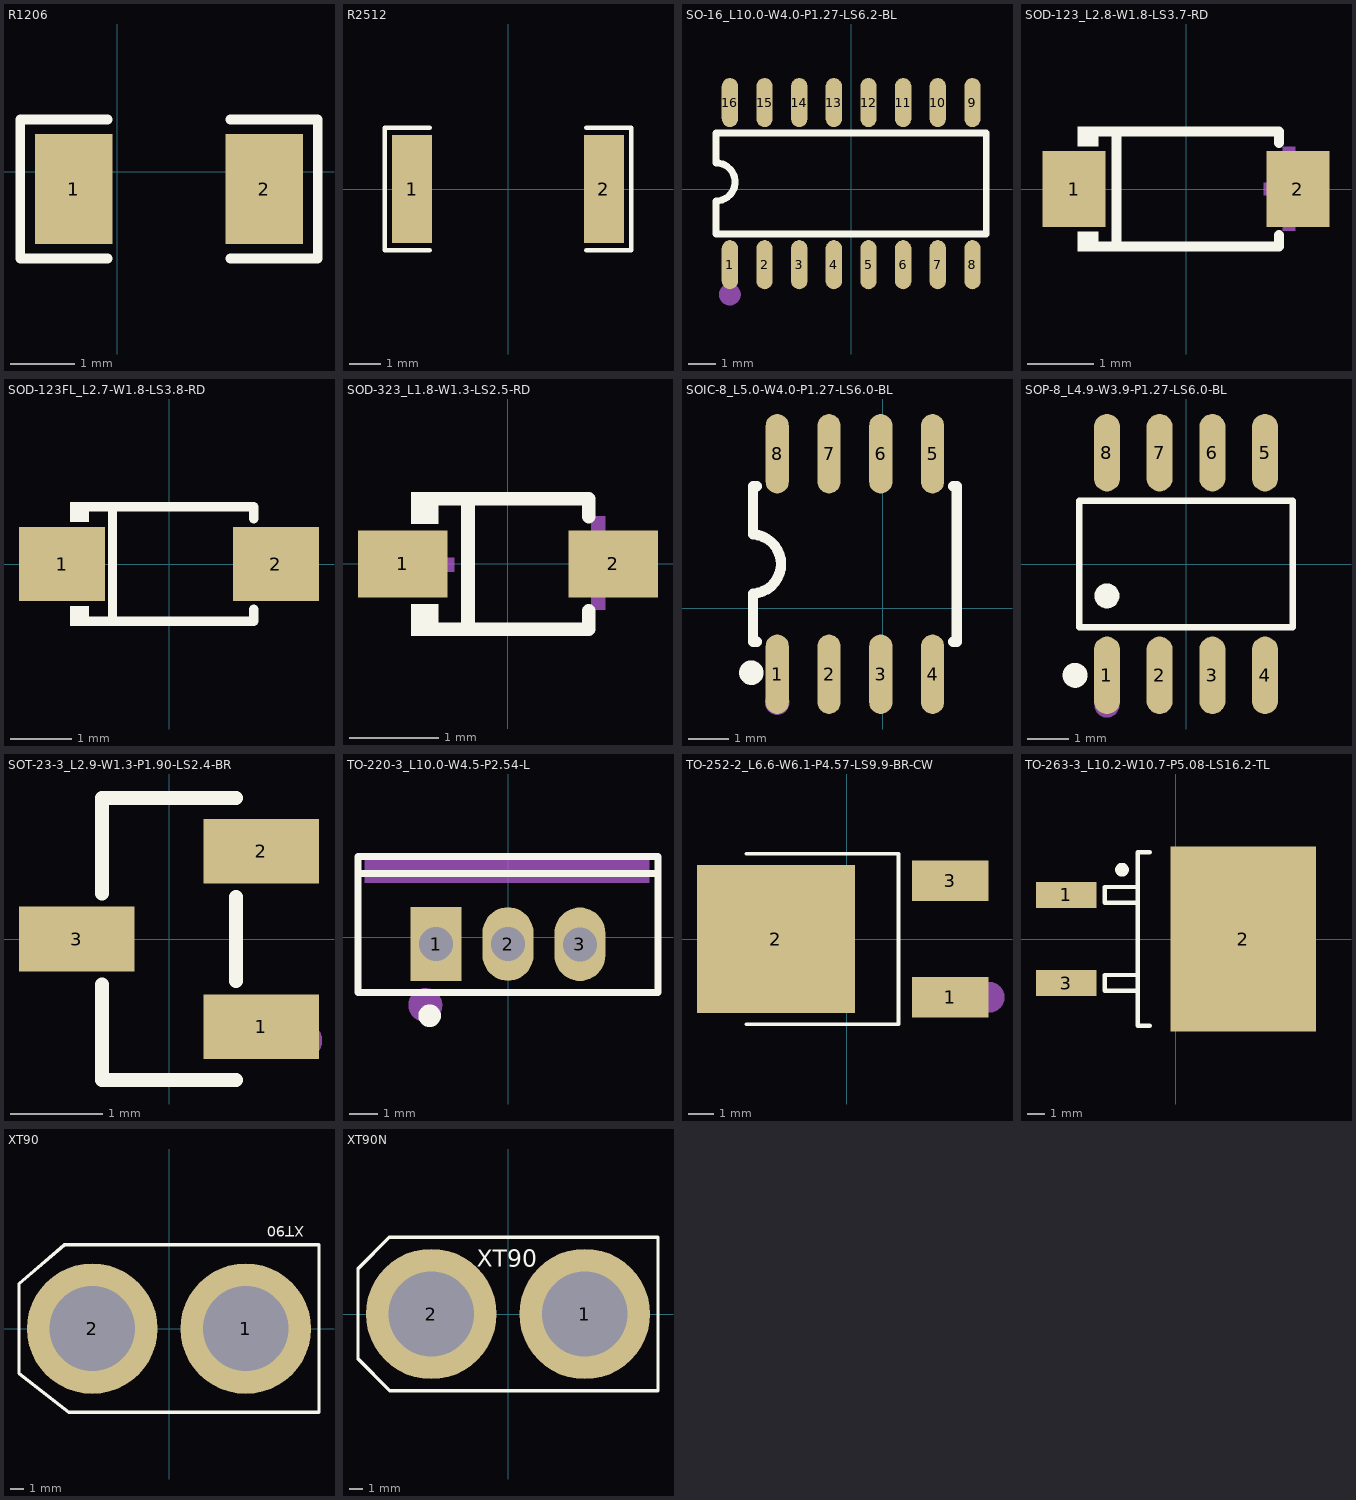
[diagram p0: the footprints below, top view; thin cyan lines are the x and y axes]
# Altium footprint library MISC84449-2.PcbLib: 30 footprints (part 2 of 2)
Each footprint in its own frame and in the unit in brackets; x right, y up, seen from the top. Pads: shape width x height; smd on the part's side, far side on the other; paste and mask are expansions set on the pad; w line width, h text height; cw(c..) or ccw(c..) is an arc to the next point about the centre after c.

## R1206 [mm]
pads (2):
  rect 1.208x1.701 smd: 1(-0.678,-0.267) 2(2.279,-0.267)
Top Overlay:
  lines w0.152: -0.151,-1.346 -1.511,-1.346 -1.511,0.812 -0.151,0.812 ; 1.751,-1.346 3.111,-1.346 3.111,0.812 1.751,0.812
Top Paste:
  region: -0.075,-1.017 -0.075,-0.656 -0.175,-0.556 -0.385,-0.556 -0.485,-0.456 -0.485,-0.078 -0.385,0.022 -0.175,0.022 -0.075,0.122 -0.075,0.484 -0.175,0.584 -1.182,0.584 -1.282,0.484 -1.282,-1.017 -1.182,-1.117 -0.175,-1.117
  region: 1.675,-1.017 1.675,-0.656 1.775,-0.556 1.986,-0.556 2.086,-0.456 2.086,-0.078 1.986,0.022 1.775,0.022 1.675,0.122 1.675,0.484 1.775,0.584 2.783,0.584 2.883,0.484 2.883,-1.017 2.783,-1.117 1.775,-1.117

## R2512 [mm]
pads (2):
  rect 1.283x3.456 smd: 1(-3.066,0) 2(3.066,0)
Top Overlay:
  lines w0.152: -2.501,-1.957 -3.936,-1.957 -3.936,1.957 -2.501,1.957 ; 2.501,-1.957 3.936,-1.957 3.936,1.957 2.501,1.957
Top Paste:
  region: 2.425,-1.628 2.425,-0.688 2.525,-0.588 2.761,-0.588 2.861,-0.488 2.861,0.488 2.761,0.588 2.525,0.588 2.425,0.688 2.425,1.628 2.525,1.728 3.608,1.728 3.708,1.628 3.708,-1.628 3.608,-1.728 2.525,-1.728
  region: -2.425,-1.628 -2.425,-0.688 -2.525,-0.588 -2.761,-0.588 -2.861,-0.488 -2.861,0.488 -2.761,0.588 -2.525,0.588 -2.425,0.688 -2.425,1.628 -2.525,1.728 -3.608,1.728 -3.708,1.628 -3.708,-1.628 -3.608,-1.728 -2.525,-1.728

## SO-16_L10.0-W4.0-P1.27-LS6.2-BL [mm]
pads (16):
  oval 0.6x1.8 smd: 1(-4.444,-2.776) 2(-3.174,-2.776) 3(-1.904,-2.776) 4(-0.634,-2.776) 5(0.636,-2.776) 6(1.906,-2.776) 7(3.176,-2.776) 8(4.446,-2.776) 9(4.446,3.168) 10(3.176,3.168) 11(1.906,3.168) 12(0.636,3.168) 13(-0.634,3.168) 14(-1.904,3.168) 15(-3.174,3.168) 16(-4.444,3.168)
Top Overlay:
  lines w0.254: -4.952,0.958 cw(c-4.952,0.26) -4.952,-0.439 -4.952,-1.654 -4.949,-1.654 4.952,-1.654 4.952,2.046 -4.949,2.046 -4.949,0.958
Mechanical 15:
  circle w0.4: c-4.444,-3.868 r0.2

## SOD-123_L2.8-W1.8-LS3.7-RD [mm]
pads (2):
  rect 0.95x1.15 smd: 1(-1.693,0) 2(1.693,0)
Top Overlay:
  region: -1.33,0.942 -1.33,0.647 -1.635,0.647 -1.635,0.942
  region: -1.33,-0.942 -1.33,-0.647 -1.635,-0.647 -1.635,-0.942
  lines w0.152: -1.406,-0.866 1.406,-0.866 1.406,-0.698 ; -1.406,0.866 1.406,0.866 1.406,0.698 ; -1.049,-0.866 -1.049,0.866
Mechanical 15:
  region: -2.03,0.095 -2.03,-0.095 -1.272,-0.095 -1.272,0.095
  region: 1.935,0.098 1.935,-0.092 1.177,-0.092 1.177,0.098
  region: 1.651,0.635 1.651,-0.629 1.461,-0.629 1.461,0.635

## SOD-123FL_L2.7-W1.8-LS3.8-RD [mm]
pads (2):
  rect 1.4x1.2 smd: 1(-1.735,0) 2(1.735,0)
Top Overlay:
  region: -1.3,1.002 -1.3,0.682 -1.605,0.682 -1.605,1.002
  region: -1.3,-1.002 -1.3,-0.682 -1.605,-0.682 -1.605,-1.002
  lines w0.152: -1.376,-0.926 1.376,-0.926 1.376,-0.733 ; -1.376,0.926 1.376,0.926 1.376,0.733 ; -0.917,-0.876 -0.917,0.876
Mechanical 15:
  region: -2.032,0.127 -2.032,-0.065 -1.264,-0.065 -1.264,0.127
  region: 2.035,0.096 2.035,-0.096 1.267,-0.096 1.267,0.096
  region: 1.747,-0.384 1.555,-0.384 1.555,0.384 1.747,0.384

## SOD-323_L1.8-W1.3-LS2.5-RD [mm]
pads (2):
  rect 1x0.75 smd: 1(-1.173,0) 2(1.173,0)
Top Overlay:
  region: -0.775,0.802 -0.775,0.45 -1.08,0.45 -1.08,0.802
  region: -0.775,-0.802 -0.775,-0.45 -1.08,-0.45 -1.08,-0.802
  lines w0.152: -0.851,-0.726 0.901,-0.726 0.901,-0.52 ; -0.851,0.726 0.901,0.726 0.901,0.53 ; -0.447,-0.726 -0.447,0.726
Mechanical 15:
  region: -1.225,0.07 -1.225,-0.086 -0.601,-0.086 -0.601,0.07
  region: 1.315,0.09 1.315,-0.066 0.691,-0.066 0.691,0.09
  region: 1.083,0.53 1.083,-0.51 0.927,-0.51 0.927,0.53

## SOIC-8_L5.0-W4.0-P1.27-LS6.0-BL [mm]
pads (8):
  oval 0.568x1.95 smd: 1(-2.59,-1.623) 2(-1.32,-1.623) 3(-0.05,-1.623) 4(1.22,-1.623) 5(1.22,3.787) 6(-0.05,3.787) 7(-1.32,3.787) 8(-2.59,3.787)
Top Overlay:
  circle w0.3: c-3.225,-1.585 r0.15
  lines w0.254: -3.185,1.809 -3.185,2.582 -3.185,2.987 -3.094,2.987 ; -3.18,1.809 cw(c-3.225,1.082) -3.185,0.356 -3.185,-0.418 -3.185,-0.823 -3.094,-0.823 ; 1.723,-0.823 1.815,-0.823 1.815,-0.418 1.815,2.582 1.815,2.987 1.723,2.987
Mechanical 15:
  circle w0.3: c-2.59,-2.318 r0.15

## SOP-8_L4.9-W3.9-P1.27-LS6.0-BL [mm]
pads (8):
  oval 0.63x1.865 smd: 1(-1.905,-2.682) 2(-0.635,-2.682) 3(0.635,-2.682) 4(1.905,-2.682) 5(1.905,2.682) 6(0.635,2.682) 7(-0.635,2.682) 8(-1.905,2.682)
Top Overlay:
  circle w0.3: c-1.905,-0.769 r0.15
  circle w0.3: c-2.672,-2.682 r0.15
  lines w0.152: -2.576,-1.521 -2.576,1.521 2.576,1.521 2.576,-1.521 -2.576,-1.521
Mechanical 15:
  circle w0.3: c-1.905,-3.4 r0.15

## SOT-23-3_L2.9-W1.3-P1.90-LS2.4-BR [mm]
pads (3):
  rect 1.25x0.7 smd: 1(1,-0.95) 2(1,0.95) 3(-1,0)
Top Overlay:
  lines w0.152: -0.726,-0.495 -0.726,-1.526 0.726,-1.526 ; -0.726,0.495 -0.726,1.526 0.726,1.526 ; 0.726,-0.455 0.726,0.455
Mechanical 15:
  circle w0.2: c1.46,-1.1 r0.1

## TO-220-3_L10.0-W4.5-P2.54-L [mm]
pads (3):
  rect 1.8x2.6 hole 1.2: 1(-2.54,-0.241)
  oval 1.8x2.6 hole 1.2: 2(0,-0.241) 3(2.54,-0.251)
Top Overlay:
  lines w0.254: -5.3,2.249 5.3,2.249 ; -5.301,-1.95 5.301,-1.95 5.301,2.849 -5.301,2.849 -5.301,2.843 -5.301,-1.95
  lines w0.4: -2.77,-2.576 ccw(c-2.769,-2.776) -2.767,-2.576
Mechanical 15:
  circle w0.6: c-2.921,-2.4 r0.3
  region: -5.06,2.765 -5.06,1.925 4.99,1.925 4.99,2.765

## TO-252-2_L6.6-W6.1-P4.57-LS9.9-BR-CW [mm]
pads (3):
  rect 3x1.6 smd: 1(4.06,-2.29) 3(4.06,2.29)
  rect 6.2x5.8 smd: 2(-2.788,0)
Top Overlay:
  lines w0.152: -3.949,-3.346 2.018,-3.346 2.018,3.346 -3.949,3.346
Mechanical 15:
  circle w0.6: c5.589,-2.286 r0.3

## TO-263-3_L10.2-W10.7-P5.08-LS16.2-TL [mm]
pads (3):
  rect 3.504x1.5 smd: 1(-6.325,2.54) 3(-6.325,-2.54)
  rect 8.38x10.7 smd: 2(3.888,0)
Top Overlay:
  lines w0.254: -2.213,-2.98 -4.112,-2.98 -4.113,-2.08 -2.213,-2.08 ; -2.213,2.1 -4.112,2.1 -4.112,3 -2.213,3 ; -1.513,-5 -2.213,-5 -2.213,5 -1.513,5
  lines w0.4: -3.115,3.8 cw(c-3.114,4) -3.113,3.8

## XT90 [mm]
pads (2):
  round 9.5 hole 6.2: 1(5.588,0) 2(-5.588,0)
Top Overlay:
  lines w0.254: -10.922,-3.263 -7.295,-6.096 10.922,-6.096 10.922,6.096 -7.62,6.096 -10.922,3.263 -10.922,-3.263
  text "XT90" at 9.845,7.46 h0.76

## XT90N [mm]
pads (2):
  round 9.5 hole 6.2: 1(5.588,0) 2(-5.588,0)
Top Overlay:
  lines w0.254: -10.922,-3.263 -10.922,3.084 -10.922,3.302 -8.636,5.588 10.922,5.588 10.922,-5.588 -8.597,-5.588 -10.922,-3.263
  text "XT90" at -2.286,3.439 h1.25